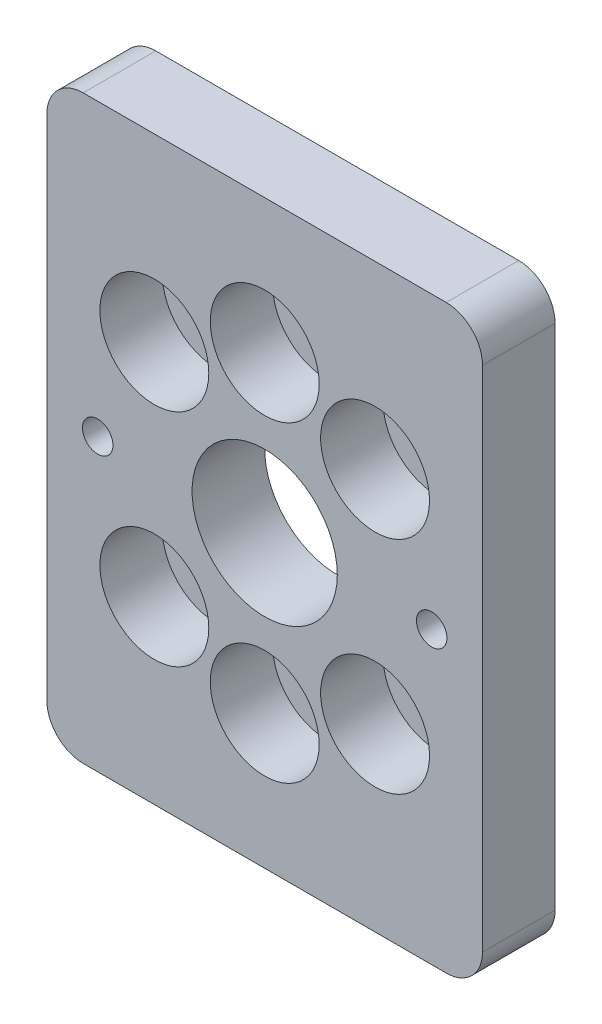
SolidWorks part; units mm, degrees
material "普通碳钢"
ref_plane "Front Plane" through (0, 0, 0) normal (0, 0, 1) x (1, 0, 0)
ref_plane "Top Plane" through (0, 0, 0) normal (0, 1, 0) x (1, 0, 0)
ref_plane "Right Plane" through (0, 0, 0) normal (1, 0, 0) x (0, 0, -1)
sketch "Sketch1" plane through (0, 0, 0) normal (0, 0, 1) x (1, 0, 0)
  line L0 (0, 91.7758) -> (0, -63.769) construction
  line L1 (-30, -40) -> (30, -40)
  line L2 (-30, -40) -> (-30, 40)
  line L3 (-30, 40) -> (30, 40)
  line L4 (30, -40) -> (30, 40)
  line L5 (-30, -40) -> (30, 40) construction
  line L6 (-30, 40) -> (30, -40) construction
  line L7 (-78.9962, 0) -> (63.9958, 0) construction
  circle A0 centre (0, 0) radius 10
  circle A1 centre (-23, 0) radius 2
  circle A2 centre (23, 0) radius 2
  point P0 (0, 0)
  dimension "D3" = 20
  dimension "D5" = 4
  dimension "D1" = 80
  dimension "D2" = 60
  dimension "D4" = 46
extrude "Boss-Extrude1" add sketch "Sketch1" along normal blind 10 contours L3 L4 L1 L2
hole_wizard "M5 Tapped Hole1" positions "Sketch2" profile "Sketch3" tap size "M5" standard "ISO" end condition through all
sketch "Sketch2" plane through (0, 0, 10) normal (0, 0, 1) x (1, 0, 0)
  point P0 (-23, 0)
  point P3 (23, 0)
sketch "Sketch3" plane through (-23, 0, 10) normal (1, 0, 0) x (0, -1, 0)
  line L0 (0, 0) -> (0, 10)
  line L1 (0, 10) -> (2.1, 10)
  line L2 (2.1, 10) -> (2.1, 0)
  line L5 (2.1, 0) -> (0, 0)
  line L11 (0, -6.35) -> (0, 107.95) construction
  dimension "通孔螺纹孔钻头直径" = 4.2
  dimension "通孔螺纹孔钻头深度" = 10
cosmetic thread "Cosmetic thread1" parameters "D2"=5
cosmetic thread "Cosmetic thread2" parameters "D2"=5
hole_wizard "CBORE for M8 Hex Socket Head Cap Screw1" positions "Sketch4" profile "Sketch5" counterbore size "M8" standard "ISO" end condition through all
sketch "Sketch4" plane through (0, 0, 10) normal (0, 0, 1) x (1, 0, 0)
  point P0 (0, 21.5)
  dimension "D1" = 21.5
sketch "Sketch5" plane through (0, 21.5, 10) normal (1, 0, 0) x (0, -1, 0)
  line L0 (0, 0) -> (0, 10)
  line L1 (0, 10) -> (4.5, 10)
  line L3 (4.5, 10) -> (4.5, 8.6)
  line L4 (4.5, 8.6) -> (7.5, 8.6)
  line L5 (7.5, 8.6) -> (7.5, 0)
  line L7 (7.5, 0) -> (0, 0)
  line L11 (0, -6.35) -> (0, 107.95) construction
  dimension "通孔孔直径" = 9
  dimension "通孔孔深度" = 10
  dimension "柱形沉头孔直径" = 15
  dimension "柱形沉头孔深度" = 8.6
pattern_circular "CirPattern1" count 8 over 360 about axis through (0, 0, 0) along (0, 0, 1) skipping 2, 6 of "CBORE for M8 Hex Socket Head Cap Screw1"
fillet "Fillet1" radius 5 4 edges at (30, -40, 5) (-30, -40, 5) (-30, 40, 5) (30, 40, 5)
